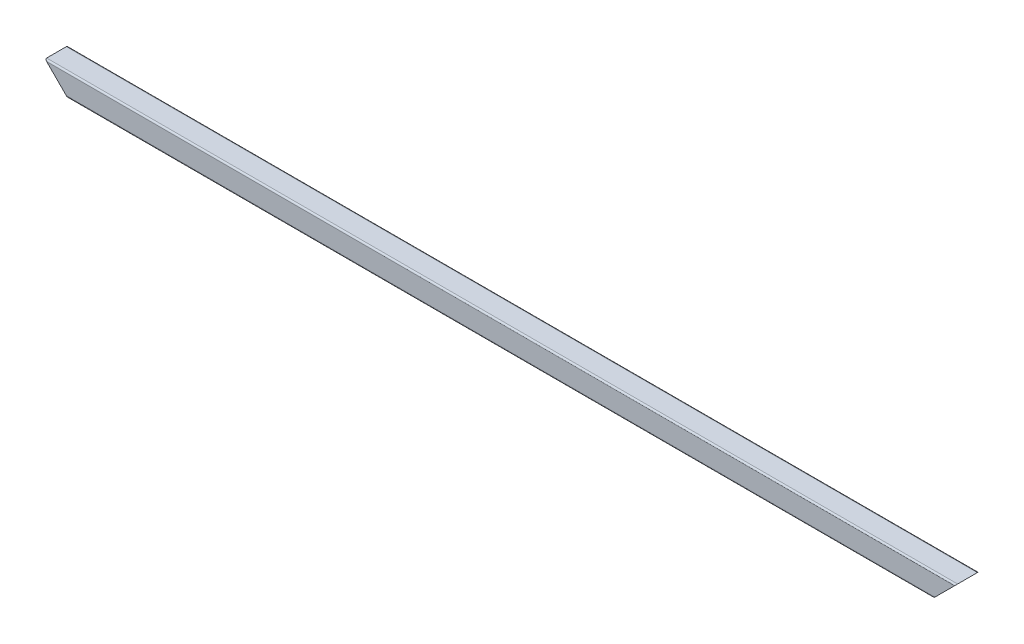
from build123d import *

# Parameters (mm, degrees)
GB_6728_1986_150_X_150_X_5_1_DEPTH = 6000
CUT_EXTRUDE_1_DEPTH                = 3005.683843602


with BuildPart() as part:
    # Sketch1 → Gb／6728-1986方形空心型钢 150 X 150 X 5(1) (new body)
    with BuildSketch(Plane.YZ.offset(-3000)):
        with BuildLine():
            Line((-65, -75), (65, -75))
            ThreePointArc((65, -75), (72.071067812, -72.071067812), (75, -65))
            Line((75, -65), (75, 65))
            ThreePointArc((75, 65), (72.071067812, 72.071067812), (65, 75))
            Line((65, 75), (-65, 75))
            ThreePointArc((-65, 75), (-72.071067812, 72.071067812), (-75, 65))
            Line((-75, 65), (-75, -65))
            ThreePointArc((-75, -65), (-72.071067812, -72.071067812), (-65, -75))
        make_face()
        with BuildLine():
            Line((-65, -70), (65, -70))
            ThreePointArc((65, -70), (68.535533906, -68.535533906), (70, -65))
            Line((70, -65), (70, 65))
            ThreePointArc((70, 65), (68.535533906, 68.535533906), (65, 70))
            Line((65, 70), (-65, 70))
            ThreePointArc((-65, 70), (-68.535533906, 68.535533906), (-70, 65))
            Line((-70, 65), (-70, -65))
            ThreePointArc((-70, -65), (-68.535533906, -68.535533906), (-65, -70))
        make_face(mode=Mode.SUBTRACT)
    extrude(amount=GB_6728_1986_150_X_150_X_5_1_DEPTH)

    # 草图6 → 切除-拉伸1 (cut, through all)
    with BuildSketch(Plane(origin=(0, 0, -75), x_dir=(-1, 0, 0), z_dir=(0, 0, -1))):
        Polygon((3000, 75), (3000, -75), (2850, -75), align=None)
        Polygon((-2850, -75), (-3000, 75), (-3000, -75), align=None)
    extrude(amount=-CUT_EXTRUDE_1_DEPTH, mode=Mode.SUBTRACT)


solid = part.part
